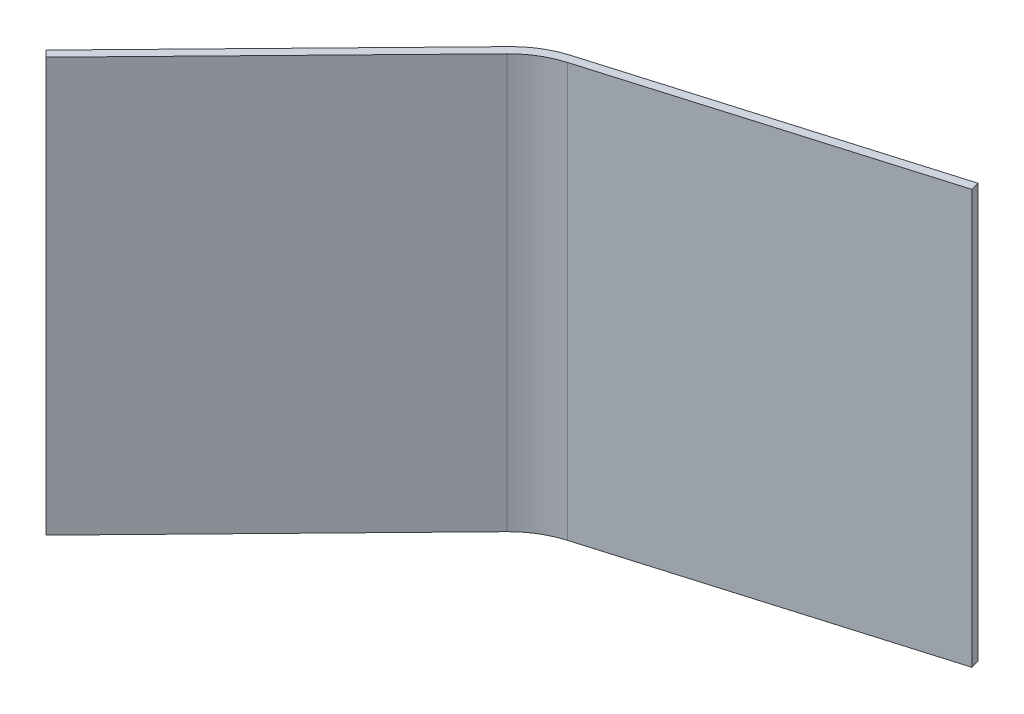
SolidWorks part; units mm, degrees
ref_plane "Front Plane" through (0, 0, 0) normal (0, 0, 1) x (1, 0, 0)
ref_plane "Top Plane" through (0, 0, 0) normal (0, 1, 0) x (1, 0, 0)
ref_plane "Right Plane" through (0, 0, 0) normal (1, 0, 0) x (0, 0, -1)
sketch "Sketch1" plane through (0, 0, 0) normal (0, 1, 0) x (1, 0, 0)
  line L0 (0, 0) -> (279.1362, 286.5013)
  line L1 (279.1362, 286.5013) -> (662.7315, 399.8798)
  line L2 (-7.1625, 6.9784) -> (273.7966, 295.3507)
  line L3 (273.7966, 295.3507) -> (659.897, 409.4696)
  line L4 (-7.1625, 6.9784) -> (0, 0)
  line L5 (659.897, 409.4696) -> (662.7315, 399.8798)
  dimension "D1" = 150.72
  dimension "D2" = 400
  dimension "D3" = 400
  dimension "D4" = 10
extrude "Boss-Extrude1" add sketch "Sketch1" along normal blind 475
fillet "Fillet1" radius 100 2 edges at (279.1362, 237.5, -286.5013) (273.7966, 237.5, -295.3507)
